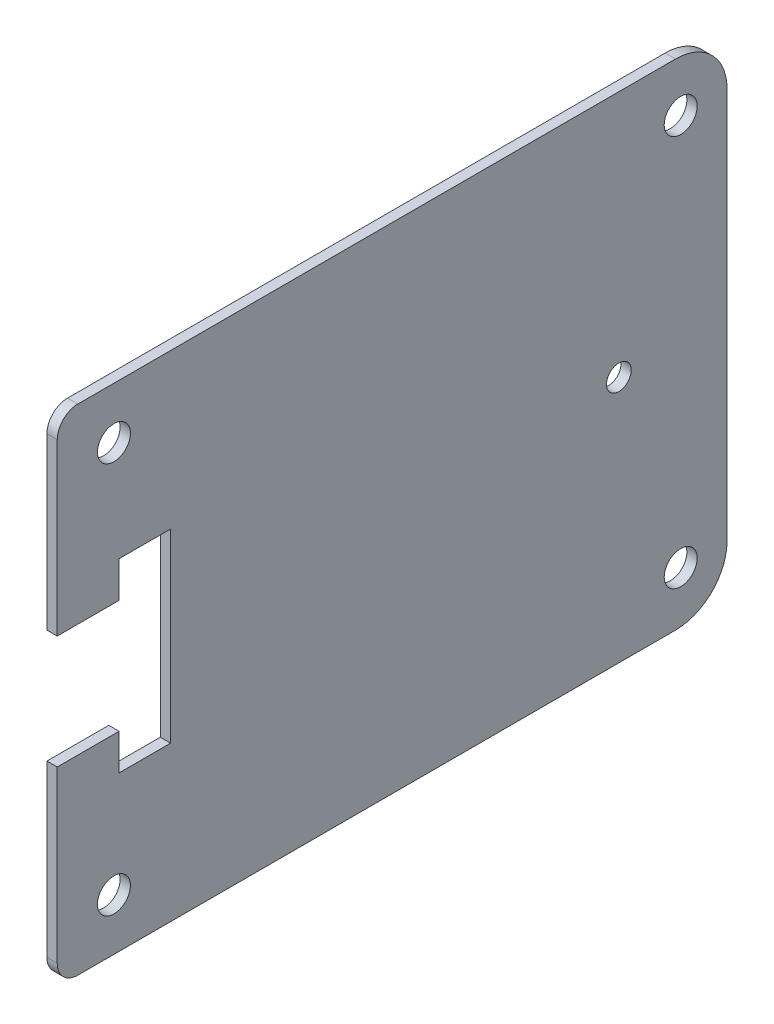
SolidWorks part; units mm, degrees
material "不锈钢201"
ref_plane "前视基准面" through (0, 0, 0) normal (0, 0, 1) x (1, 0, 0)
ref_plane "上视基准面" through (0, 0, 0) normal (0, 1, 0) x (1, 0, 0)
ref_plane "右视基准面" through (0, 0, 0) normal (1, 0, 0) x (0, 0, -1)
sketch "草图1" plane through (0, 0, 0) normal (1, 0, 0) x (0, 0, -1)
  line L1 (-32.5, 24) -> (32.5, 24)
  line L2 (-32.5, 24) -> (-32.5, -24)
  line L3 (-32.5, -24) -> (32.5, -24)
  line L4 (32.5, 24) -> (32.5, -24)
  line L5 (-32.5, 24) -> (32.5, -24) construction
  line L6 (-32.5, -24) -> (32.5, 24) construction
  point P0 (0, 0)
  dimension "D1" = 48
  dimension "D2" = 65
extrude "凸台-拉伸1" add sketch "草图1" along normal blind 20
sketch "草图2" plane through (0, 0, -32.5) normal (0, 0, -1) x (-1, 0, 0)
  line L0 (0, -24) -> (0, 24) construction
  line L1 (-3, 13.55) -> (3, 13.55)
  line L2 (-3, 13.55) -> (-3, -13.55)
  line L3 (-3, -13.55) -> (3, -13.55)
  line L4 (3, 13.55) -> (3, -13.55)
  line L5 (-3, 13.55) -> (3, -13.55) construction
  line L6 (-3, -13.55) -> (3, 13.55) construction
  point P0 (0, 0)
  dimension "D1" = 27.1
  dimension "D2" = 3
extrude "切除-拉伸1" cut sketch "草图2" against normal blind 80
sketch "草图3" plane through (20, 0, 0) normal (1, 0, 0) x (0, 0, -1)
  line L0 (-26.5, -9) -> (-21.5, -9)
  line L1 (-32.5, 5.5) -> (-26.5, 5.5)
  line L2 (-32.5, 24) -> (-32.5, -24) construction
  line L3 (-26.5, 5.5) -> (-26.5, 9)
  line L4 (-26.5, 9) -> (-21.5, 9)
  line L5 (-21.5, 9) -> (-21.5, -9)
  line L6 (-26.5, -5.5) -> (-26.5, -9)
  line L7 (0, 0) -> (-37.4252, 0) construction
  line L8 (-32.5, -5.5) -> (-26.5, -5.5)
  line L9 (-32.5, 5.5) -> (-32.5, -5.5)
  point P11 (-21.5, 0)
  dimension "D1" = 5
  dimension "D2" = 6
  dimension "D3" = 9
  dimension "D4" = 5.5
extrude "切除-拉伸2" cut sketch "草图3" against normal blind 80
sketch "草图4" plane through (20, 0, 0) normal (1, 0, 0) x (0, 0, -1)
  line L0 (0, 0) -> (39.4787, 0) construction
  line L1 (32.5, -24) -> (32.5, 24) construction
  circle A0 centre (22, 0) radius 1.2
  dimension "D1" = 2.4
  dimension "D2" = 10.5
extrude "切除-拉伸3" cut sketch "草图4" against normal blind 6
chamfer "倒角2" [suppressed] distance 0.5 angle 45
hole_wizard "打孔尺寸(%根据)开槽圆柱头螺钉的类型1" positions "草图5" profile "草图6" counterbore size "M3" standard "GB" end condition through all
sketch "草图5" plane through (20, 0, 0) normal (1, 0, 0) x (0, 0, -1)
  point P0 (7.35, -10)
  point P3 (-7.65, -10)
  point P6 (-7.65, 10)
  point P17 (7.35, 10)
sketch "草图6" plane through (20, -10, -7.35) normal (0, 1, 0) x (0, 0, -1)
  line L0 (0, 0) -> (0, 20)
  line L1 (0, 20) -> (1.7, 20)
  line L3 (1.7, 20) -> (1.7, 5)
  line L4 (1.7, 5) -> (3, 5)
  line L5 (3, 5) -> (3, 0)
  line L7 (3, 0) -> (0, 0)
  line L11 (0, -6.35) -> (0, 107.95) construction
  dimension "通孔孔直径" = 3.4
  dimension "通孔孔深度" = 20
  dimension "柱形沉头孔直径" = 6
  dimension "柱形沉头孔深度" = 5
fillet "圆角1" radius 5 2 edges at (10, -24, -32.5) (10, 24, -32.5)
sketch "草图7" [suppressed] plane through (20, 0, 0) normal (1, 0, 0) x (0, 0, -1)
  circle A0 centre (22, 0) radius 0.5
  dimension "D1" = 1
extrude "切除-拉伸4" [suppressed] cut sketch "草图7" against normal blind 28
sketch "草图8" [suppressed] plane through (3, 0, 0) normal (-1, 0, 0) x (0, 0, 1)
  circle A0 centre (-22, 0) radius 5.05
  dimension "D1" = 10.1
extrude "切除-拉伸5" [suppressed] cut sketch "草图8" against normal blind 5
sketch "草图9" plane through (0, 24, 0) normal (0, 1, 0) x (1, 0, 0)
  line L0 (20, 27.5) -> (20, -32.5) construction
  line L1 (-0.0821, 41.997) -> (19, 41.997)
  line L2 (-0.0821, 41.997) -> (-0.0821, -42.1601)
  line L3 (-0.0821, -42.1601) -> (19, -42.1601)
  line L4 (19, 41.997) -> (19, -42.1601)
  dimension "D1" = 1
extrude "切除-拉伸6" cut sketch "草图9" against normal blind 120
sketch "草图10" plane through (19, 0, 0) normal (-1, 0, 0) x (0, 0, 1)
  line L1 (-11.7057, 14.4772) -> (13.3103, 14.4772)
  line L2 (-11.7057, 14.4772) -> (-11.7057, -15.79)
  line L3 (-11.7057, -15.79) -> (13.3103, -15.79)
  line L4 (13.3103, 14.4772) -> (13.3103, -15.79)
extrude "凸台-拉伸2" add sketch "草图10" against normal up to surface (1 mm away) up to face at (20, -10, -10.35)
sketch "草图11" plane through (19, 0, 0) normal (-1, 0, 0) x (0, 0, 1)
  line L0 (0, 0) -> (-36.7503, 0) construction
  line L1 (0, 31.0315) -> (0, -41.1983) construction
  circle A0 centre (-28, 19) radius 1.6
  circle A1 centre (-28, -19) radius 1.6
  circle A2 centre (27, -19) radius 1.6
  circle A3 centre (27, 19) radius 1.6
  point P13 (0, 0)
  point P14 (0, 0)
  dimension "D1" = 3.2
  dimension "D2" = 28
  dimension "D3" = 0
  dimension "D5" = 27
extrude "切除-拉伸7" cut sketch "草图11" against normal blind 120
fillet "圆角2" radius 2 2 edges at (19.5, 24, 32.5) (19.5, -24, 32.5)
